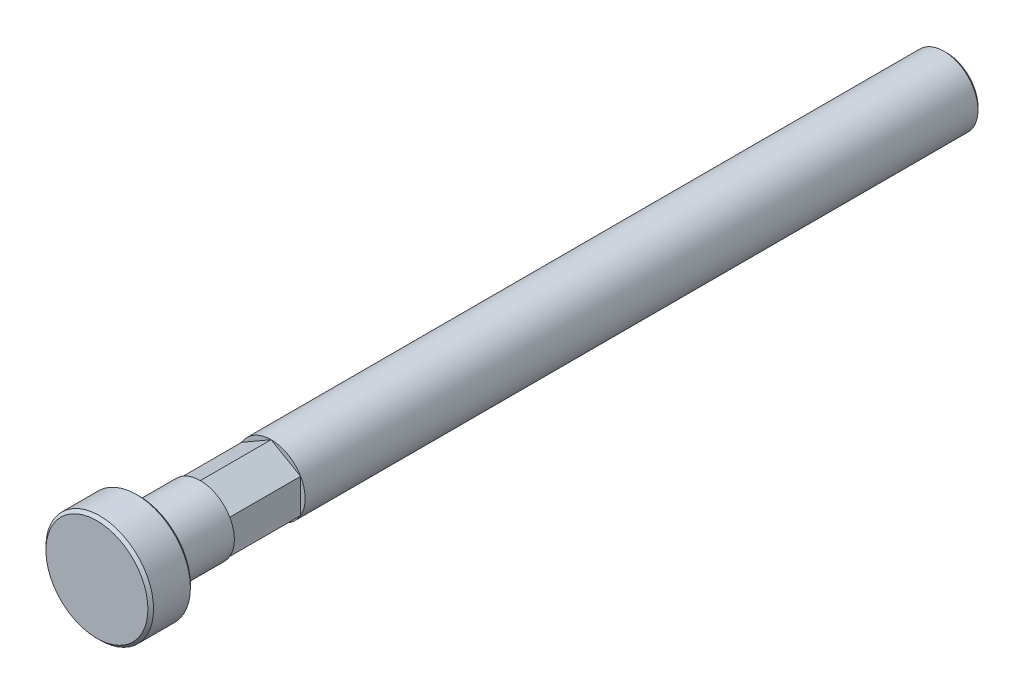
SolidWorks part; units mm, degrees
material "Q235"
ref_plane "Front Plane" through (0, 0, 0) normal (0, 0, 1) x (1, 0, 0)
ref_plane "Top Plane" through (0, 0, 0) normal (0, 1, 0) x (1, 0, 0)
ref_plane "Right Plane" through (0, 0, 0) normal (1, 0, 0) x (0, 0, -1)
sketch "Sketch1" plane through (0, 0, 0) normal (0, 0, 1) x (1, 0, 0)
  line L1 (20.7846, 12) -> (0, 24)
  line L2 (0, 24) -> (-20.7846, 12)
  line L3 (-20.7846, 12) -> (-20.7846, -12)
  line L4 (-20.7846, -12) -> (0, -24)
  line L5 (0, -24) -> (20.7846, -12)
  line L6 (20.7846, -12) -> (20.7846, 12)
  circle A0 centre (0, 0) radius 24 construction
  dimension "D1" = 48
extrude "Boss-Extrude1" add sketch "Sketch1" along normal blind 50
sketch "Sketch2" plane through (0, 0, 50) normal (0, 0, 1) x (1, 0, 0)
  circle A0 centre (0, 0) radius 24
  dimension "D1" = 48
extrude "Boss-Extrude2" add sketch "Sketch2" along normal blind 43
sketch "Sketch3" plane through (0, 0, 93) normal (0, 0, 1) x (1, 0, 0)
  circle A0 centre (0, 0) radius 38
  dimension "D1" = 76
extrude "Boss-Extrude3" add sketch "Sketch3" along normal blind 30
sketch "Sketch4" plane through (0, 0, 0) normal (0, 0, -1) x (-1, 0, 0)
  circle A0 centre (0, 0) radius 24
  dimension "D1" = 48
extrude "Boss-Extrude4" add sketch "Sketch4" along normal blind 477
cosmetic thread "Cosmetic Thread1" parameters "D2"=29
chamfer "Chamfer1" distance 2 angle 45 3 edges at (38, 0, 93) (38, 0, 123) (-24, 0, -477)
